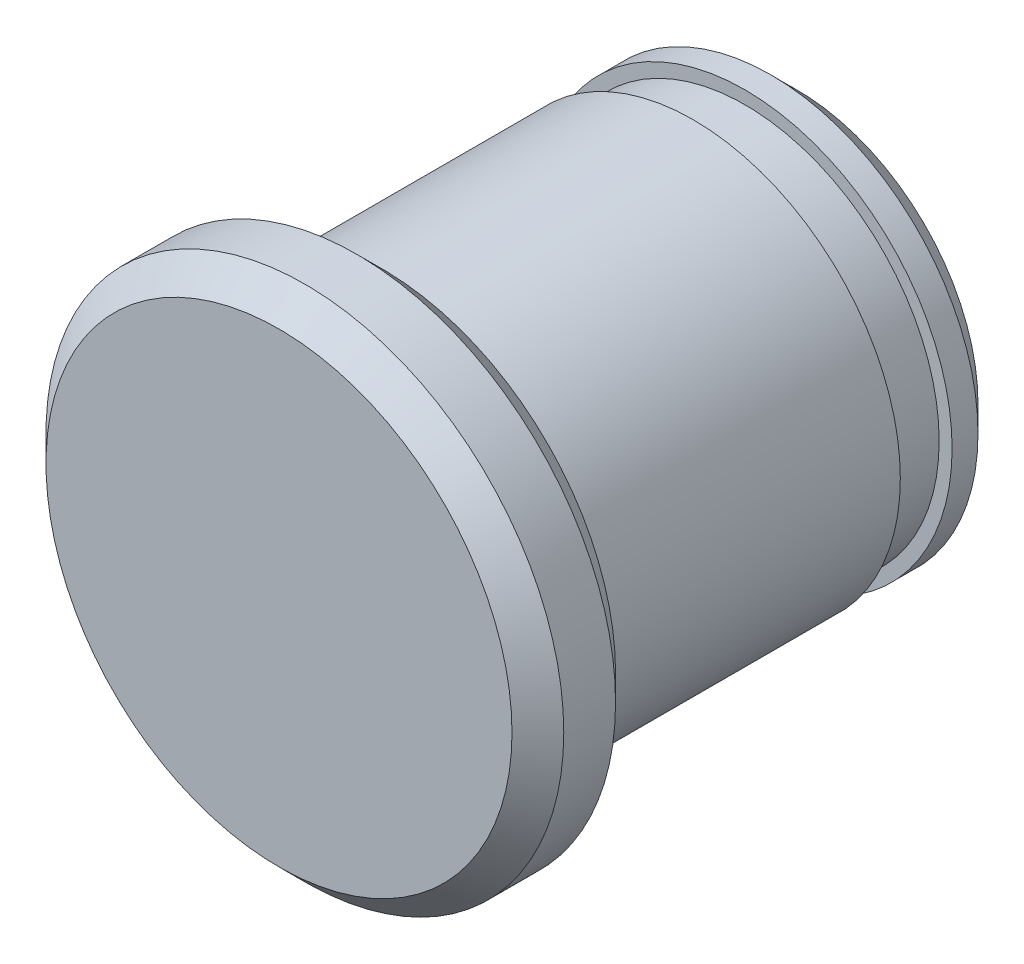
SolidWorks part; units mm, degrees
ref_plane "Front Plane" through (0, 0, 0) normal (0, 0, 1) x (1, 0, 0)
ref_plane "Top Plane" through (0, 0, 0) normal (0, 1, 0) x (1, 0, 0)
ref_plane "Right Plane" through (0, 0, 0) normal (1, 0, 0) x (0, 0, -1)
other "Configuration Table"
sketch "Sketch1" plane through (0, 0, 0) normal (0, 0, 1) x (1, 0, 0)
  circle A0 centre (0, 0) radius 4
  dimension "D1" = 8
extrude "Boss-Extrude1" add sketch "Sketch1" along normal blind 1
sketch "Sketch2" plane through (0, 0, 1) normal (0, 0, 1) x (1, 0, 0)
  circle A0 centre (0, 0) radius 3.75
  dimension "D1" = 7.5
extrude "Boss-Extrude2" add sketch "Sketch2" along normal blind 1
sketch "Sketch3" plane through (0, 0, 2) normal (0, 0, 1) x (1, 0, 0)
  circle A0 centre (0, 0) radius 4
  dimension "D1" = 8
extrude "Boss-Extrude3" add sketch "Sketch3" along normal blind 6
sketch "Sketch4" plane through (0, 0, 8) normal (0, 0, 1) x (1, 0, 0)
  circle A0 centre (0, 0) radius 5
  dimension "D1" = 10
extrude "Boss-Extrude4" add sketch "Sketch4" along normal blind 2
chamfer "Chamfer1" distance 0.5 angle 45 3 edges at (4, 0, 0) (5, 0, 8) (5, 0, 10)
